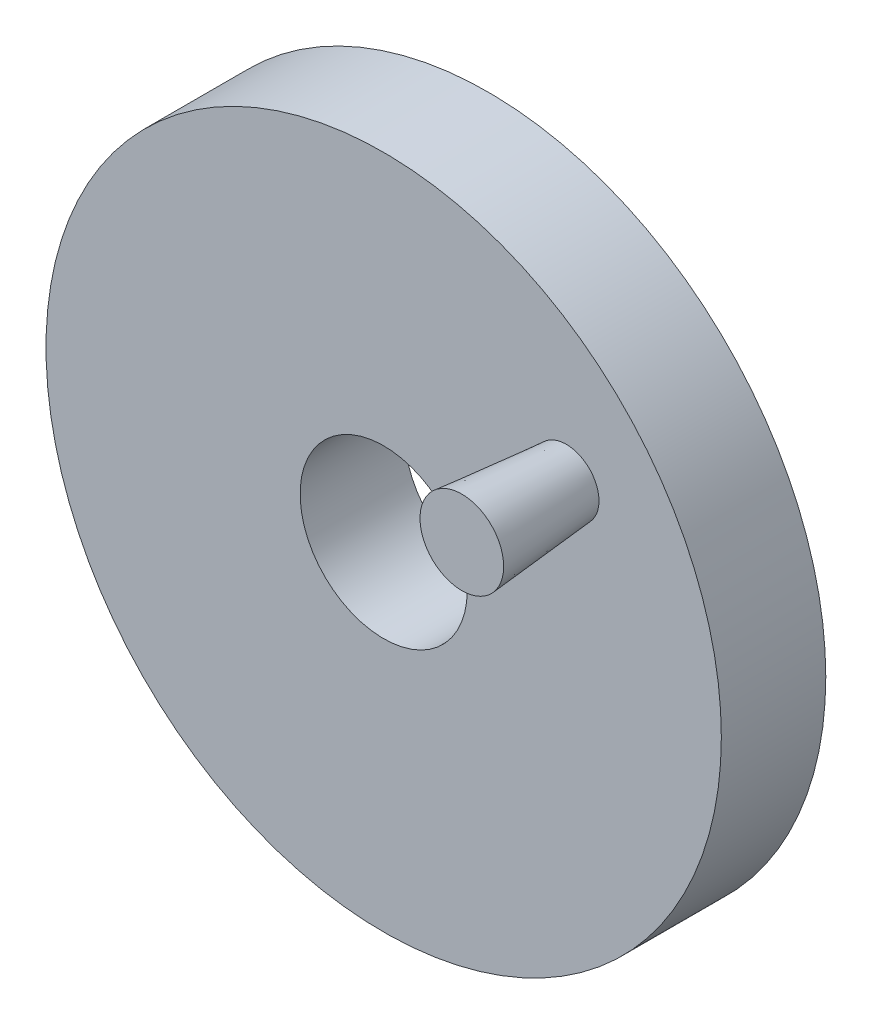
from build123d import *

# Parameters (mm, degrees)
SKETCH1_R           = 32.327609768
SKETCH1_R_2         = 8
BOSS_EXTRUDE1_DEPTH = 10
SKETCH2_R           = 3.129710108
BOSS_EXTRUDE2_DEPTH = 10
BOSS_EXTRUDE2_DRAFT = -5


with BuildPart() as part:
    # Sketch1 → Boss-Extrude1 (new body)
    with BuildSketch(Plane.XY):
        with Locations((0, -208.707425476)):
            Circle(SKETCH1_R)
        with Locations((0, -208.707425476)):
            Circle(SKETCH1_R_2, mode=Mode.SUBTRACT)
    extrude(amount=-BOSS_EXTRUDE1_DEPTH)


with BuildPart() as boss_extrude2_tool:
    # Sketch2 → Boss-Extrude2 (with draft: the straight prism first)
    with BuildSketch(Plane.XY):
        with Locations((17.482051152, -194.976936722)):
            Circle(SKETCH2_R)
    extrude(amount=BOSS_EXTRUDE2_DEPTH)
    # Boss-Extrude2: the draft: its side faces are tilted about the plane it starts from
    boss_extrude2_sides = [boss_extrude2_tool.faces().sort_by_distance(p)[0] for p in [
        (14.352341045, -194.976936722, 5),
    ]]
    draft(boss_extrude2_sides, Plane.XY, BOSS_EXTRUDE2_DRAFT)


with BuildPart() as part_1:
    add(part.part)

    # Boss-Extrude2: add boss_extrude2_tool
    add(boss_extrude2_tool.part)


solid = part_1.part
